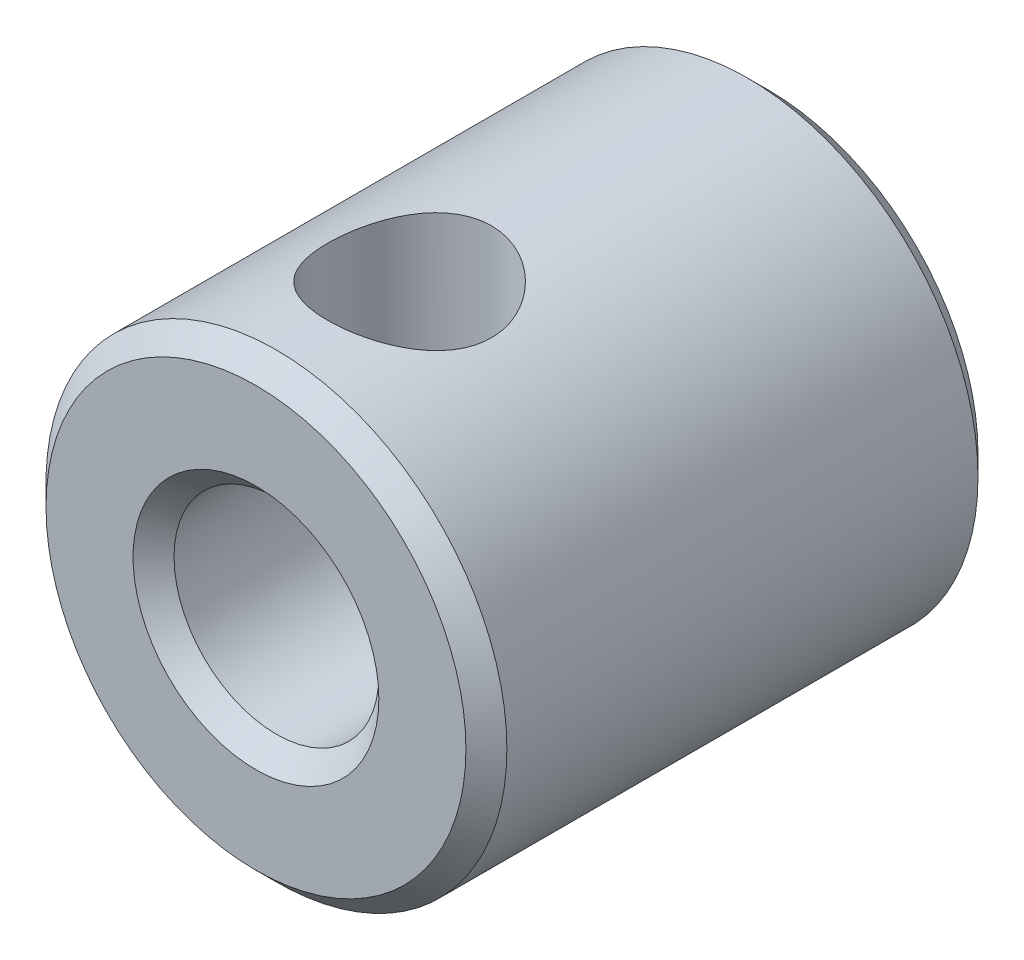
from build123d import *

# Parameters (mm, degrees)
SKETCH1_R           = 2.25
SKETCH1_R_2         = 1
BOSS_EXTRUDE1_DEPTH = 2.5
CHAMFER1_SIZE       = 0.2
SKETCH2_W           = 0.8
SKETCH2_H           = 2.25


with BuildPart() as part:
    # Sketch1 → Boss-Extrude1 (new, symmetric)
    with BuildSketch(Plane.XY):
        Circle(SKETCH1_R)
        Circle(SKETCH1_R_2, mode=Mode.SUBTRACT)
    extrude(amount=BOSS_EXTRUDE1_DEPTH, both=True)

    # Chamfer1
    chamfer1_edges = [part.edges().sort_by_distance(p)[0] for p in [
        (-2.25, 0, -2.5),
        (-2.25, 0, 2.5),
        (-1, 0, -2.5),
        (-1, 0, 2.5),
    ]]
    chamfer(chamfer1_edges, length=CHAMFER1_SIZE)

    # Sketch2 → M2 Tapped Hole1 (revolve, cut)
    with BuildSketch(Plane(origin=(0, 0, 1), x_dir=(0, 0, -1), z_dir=(1, 0, 0))):
        with Locations((0.4, 1.125)):
            Rectangle(SKETCH2_W, SKETCH2_H)
    revolve(axis=Axis((0, -6.35, 1), (0, 1, 0)), mode=Mode.SUBTRACT)


solid = part.part
